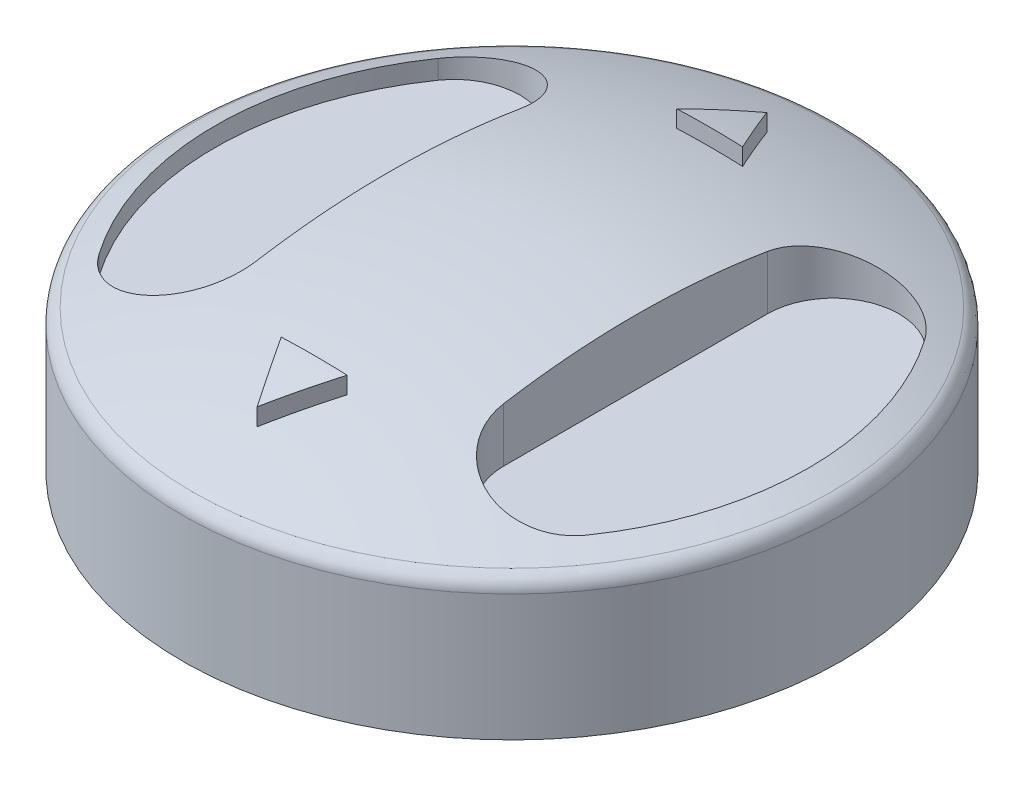
SolidWorks part; units mm, degrees
ref_plane "Front Plane" through (0, 0, 0) normal (0, 0, 1) x (1, 0, 0)
ref_plane "Top Plane" through (0, 0, 0) normal (0, 1, 0) x (1, 0, 0)
ref_plane "Right Plane" through (0, 0, 0) normal (1, 0, 0) x (0, 0, -1)
sketch "Sketch1" plane through (0, 0, 0) normal (0, 0, 1) x (1, 0, 0)
  line L0 (20, 8.3258) -> (20, 0)
  line L1 (20, 0) -> (0, 0)
  line L2 (0, 0) -> (0, 12.5) construction
  line L3 (0, 12.5) -> (0, 0)
  arc A0 (0, 12.5) -> (20, 8.3258) centre (0, -37.5) cw
  dimension "D2" = 50
  dimension "D1" = 20
  dimension "D3" = 12.5
revolve "Revolve1" add sketch "Sketch1" angle 360 about L2
fillet "Fillet1" radius 1 1 edges at (20, 8.3258, 0)
sketch "Sketch2" plane through (0, 0, 0) normal (0, -1, 0) x (1, 0, 0)
  circle A0 centre (0, 0) radius 10
  dimension "D1" = 20
extrude "Boss-Extrude1" add sketch "Sketch2" along normal blind 2.5
ref_plane "Plane1" through (0, 8, 0) normal (0, -1, 0) x (-1, 0, 0)
sketch "Sketch3" plane through (0, 8, 0) normal (0, -1, 0) x (-1, 0, 0)
  line L0 (7.5, 8) -> (7.5, -8)
  line L1 (0, 8.25) -> (0, -8.25) construction
  line L2 (-7.5, 8) -> (-7.5, -8)
  arc A0 (14.7742, -10.2821) -> (14.7742, 10.2821) centre (0, 0) ccw
  arc A1 (14.7742, 10.2821) -> (7.5, 8) centre (11.4951, 8) ccw
  arc A2 (7.5, -8) -> (14.7742, -10.2821) centre (11.4951, -8) ccw
  arc A3 (-7.5, -8) -> (-14.7742, -10.2821) centre (-11.4951, -8) cw
  arc A4 (-14.7742, -10.2821) -> (-14.7742, 10.2821) centre (0, 0) cw
  arc A5 (-14.7742, 10.2821) -> (-7.5, 8) centre (-11.4951, 8) cw
  dimension "D1" = 36
  dimension "D2" = 7.5
  dimension "D3" = 8
  dimension "D4" = 8
extrude "Cut-Extrude1" cut sketch "Sketch3" against normal blind 10.5
sketch "Sketch4" plane through (0, 0, 0) normal (1, 0, 0) x (0, 0, -1)
  line L0 (0, 0) -> (0, 17.5) construction
  line L1 (0, 17.5) -> (0, 13.5)
  line L2 (0, 12.5) -> (0, 17.5) construction
  arc A0 (19.3878, 8.5881) -> (-19.3878, 8.5881) centre (0, -37.5) ccw construction
  arc A1 (18.8679, 8.8034) -> (0, 12.5) centre (0, -37.5) ccw construction
  arc A2 (20.7547, 13.4337) -> (0, 17.5) centre (0, -37.5) ccw
  arc A3 (20.7547, 13.4337) -> (-21.3265, 13.1969) centre (0, -37.5) ccw construction
  arc A4 (18.8679, 8.8034) -> (-19.3878, 8.5881) centre (0, -37.5) ccw construction
  arc A5 (20.7547, 13.4337) -> (19.2453, 9.7294) centre (20, 11.5816) cw
  arc A6 (19.2453, 9.7294) -> (0, 13.5) centre (0, -37.5) ccw
  dimension "D2" = 1
  dimension "D1" = 5
sketch "Sketch5" plane through (0, 0, 0) normal (0, -1, 0) x (1, 0, 0)
  line L0 (2, -12) -> (0, -15.4641)
  line L1 (0, -18.8679) -> (0, 0) construction
  line L2 (0, -15.4641) -> (-2, -12)
  line L3 (-2, -12) -> (2, -12)
  line L4 (8.8, 0) -> (-8.8, 0) construction
  line L5 (2, 12) -> (0, 15.4641)
  line L6 (0, 15.4641) -> (-2, 12)
  line L7 (-2, 12) -> (2, 12)
  dimension "D1" = 4
  dimension "D2" = 12
extrude "Boss-Extrude2" add sketch "Sketch5" against normal blind 13.5
revolve "Cut-Revolve3" cut sketch "Sketch4" angle 360 about L0
